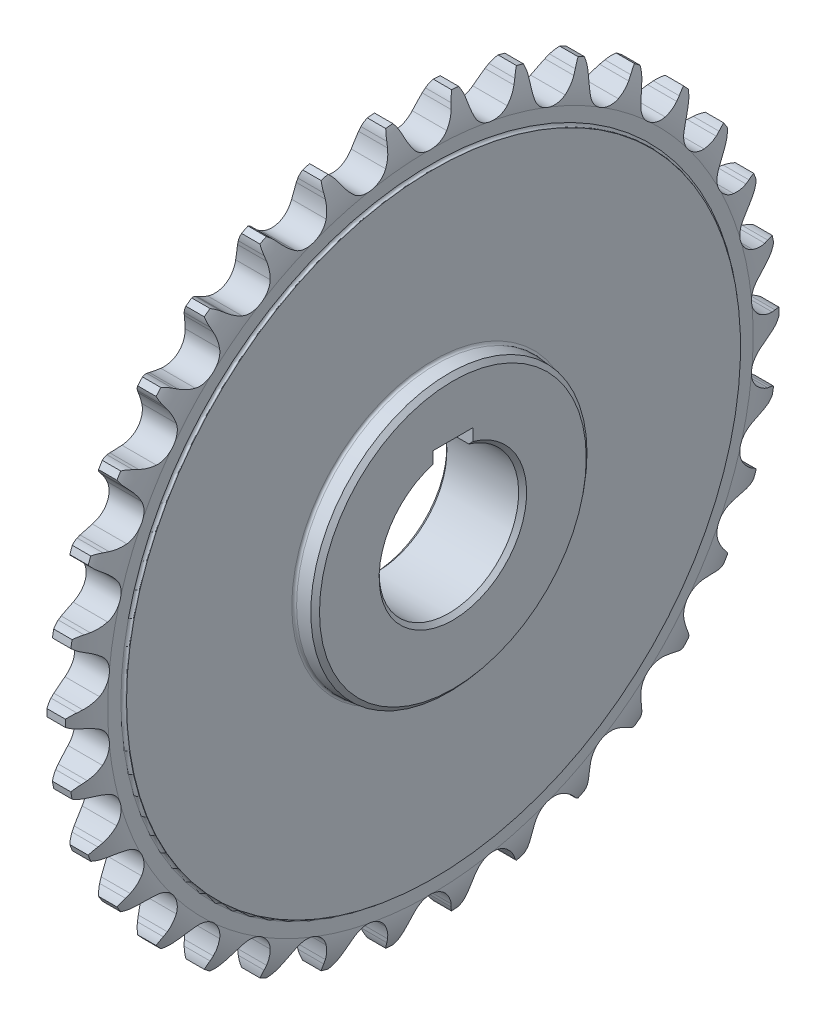
from build123d import *
from OCP.BRepFilletAPI import BRepFilletAPI_MakeChamfer

# Parameters (mm, degrees)
CUT_EXTRUDE_1_DEPTH      = 5.15
PATTERN_CIRCULAR_1_COUNT = 34
SKETCH_4_W               = 10
SKETCH_4_H               = 4.029490121
CUT_EXTRUDE_2_DEPTH      = 128.262907118
FILLET_1_R               = 0.635
CHAMFER_1_SIZE           = 1
CHAMFER_1_SIZE2          = 1.100062868


with BuildPart() as part:
    # 草图1 → 旋转1 (revolve)
    with BuildSketch(Plane.XY, mode=Mode.PRIVATE) as revolve_1_sk:
        with BuildLine():
            Line((-5.15, 17.5), (-5.15, 77))
            Line((-5.15, 77), (-5.006, 77))
            ThreePointArc((-5.006, 77), (-4.556987194, 77.185987194), (-4.371, 77.635))
            Line((-4.371, 77.635), (-4.371, 80.946239614))
            ThreePointArc((-4.371, 80.946239614), (-3.943611485, 85.368963147), (-2.30725, 89.5))
            Line((-2.30725, 89.5), (2.30725, 89.5))
            ThreePointArc((2.30725, 89.5), (3.943611485, 85.368963147), (4.371, 80.946239614))
            Line((4.371, 80.946239614), (4.371, 77.635))
            ThreePointArc((4.371, 77.635), (4.556987194, 77.185987194), (5.006, 77))
            Line((5.006, 77), (5.15, 77))
            Line((5.15, 77), (5.15, 17.5))
            Line((5.15, 17.5), (-5.15, 17.5))
        make_face()
    revolve(revolve_1_sk.sketch.rotate(Axis((-7.9375, 0, 0), (1, 0, 0)), 90), axis=Axis((-7.9375, 0, 0), (1, 0, 0)))

    # 草图2 → 切除-拉伸1 (cut, symmetric)
    with BuildSketch(Plane(origin=(0, 0, 0), x_dir=(0, 0, -1), z_dir=(1, 0, 0))):
        with BuildLine():
            Line((5.937998019, 86.258315079), (6.34124112, 87.341922018))
            ThreePointArc((6.34124112, 87.341922018), (6.78291151, 88.306679102), (7.360367351, 89.196832861))
            ThreePointArc((7.360367351, 89.196832861), (0, 89.5), (-7.360367351, 89.196832861))
            ThreePointArc((-7.360367351, 89.196832861), (-6.78291151, 88.306679102), (-6.34124112, 87.341922018))
            Line((-6.34124112, 87.341922018), (-5.937998019, 86.258315079))
            ThreePointArc((-5.937998019, 86.258315079), (-5.15256189, 84.534832792), (-4.129992057, 82.940576838))
            ThreePointArc((-4.129992057, 82.940576838), (0, 80.870839614), (4.129992057, 82.940576838))
            ThreePointArc((4.129992057, 82.940576838), (5.15256189, 84.534832792), (5.937998019, 86.258315079))
        make_face()
    cut_extrude_1 = extrude(amount=CUT_EXTRUDE_1_DEPTH, both=True, mode=Mode.SUBTRACT)

    # 阵列(圆周)1: 切除-拉伸1 ×34 about axis
    pattern_circular_1_axis = Axis((0, 0, 0), (1, 0, 0))
    for i in range(1, PATTERN_CIRCULAR_1_COUNT):
        add(cut_extrude_1.rotate(pattern_circular_1_axis, i * 360 / PATTERN_CIRCULAR_1_COUNT), mode=Mode.SUBTRACT)

    # 草图5 → 旋转2 (revolve)
    with BuildSketch(Plane.XY, mode=Mode.PRIVATE) as revolve_2_sk:
        Polygon((-10, 17.5), (10, 17.5), (10, 34.553858126), (5.15, 34.978178144), (-5.15, 34.978178144), (-10, 34.553858126), align=None)
    revolve(revolve_2_sk.sketch.rotate(Axis((0, 0, 0), (-1, 0, 0)), 90), axis=Axis((0, 0, 0), (-1, 0, 0)))

    # 草图4 → 切除-拉伸2 (cut, through all)
    with BuildSketch(Plane.ZY.offset(5.15)):
        with Locations((0, 18.785254892)):
            Rectangle(SKETCH_4_W, SKETCH_4_H)
    cut_extrude_2 = extrude(amount=-CUT_EXTRUDE_2_DEPTH, mode=Mode.SUBTRACT)

    # 镜向1: 切除-拉伸2 across plane
    add(cut_extrude_2.mirror(Plane(origin=(0, 0, 0), x_dir=(0, 0, 1), z_dir=(1, 0, 0))), mode=Mode.SUBTRACT)

    # 圆角1
    fillet_1_edges = [part.edges().sort_by_distance(p)[0] for p in [
        (-5.15, 0, 34.978178144),
        (5.15, 0, 34.978178144),
    ]]
    fillet(fillet_1_edges, radius=FILLET_1_R)

    # 倒角1: one chamfer whose edges measure the first distance from different faces: ONE call of the kernel's chamfer builder (chamfer() names one face for all edges)
    chamfer_1_edges_1 = [part.edges().sort_by_distance(p)[0] for p in [
        (-10, 0, 34.553858126),
    ]]
    chamfer_1_side_1 = [part.faces().sort_by_distance(p)[0] for p in [
        (-10, 0, 33.57652743),
    ]]
    chamfer_1_edges_2 = [part.edges().sort_by_distance(p)[0] for p in [
        (10, 0, 34.553858126),
    ]]
    chamfer_1_side_2 = [part.faces().sort_by_distance(p)[0] for p in [
        (7.864828052, 0, 34.740661466),
    ]]
    chamfer_1_edges_3 = [part.edges().sort_by_distance(p)[0] for p in [
        (10, -17.5, 0),
        (-10, -17.5, 0),
    ]]
    chamfer_1 = BRepFilletAPI_MakeChamfer(part.part.solid().wrapped)
    for e in chamfer_1_edges_1:
        chamfer_1.Add(CHAMFER_1_SIZE, CHAMFER_1_SIZE2, e.wrapped, chamfer_1_side_1[0].wrapped)  # the first distance lies on this face
    for e in chamfer_1_edges_2:
        chamfer_1.Add(CHAMFER_1_SIZE, CHAMFER_1_SIZE2, e.wrapped, chamfer_1_side_2[0].wrapped)  # the first distance lies on this face
    for e in chamfer_1_edges_3:
        chamfer_1.Add(CHAMFER_1_SIZE, e.wrapped)
    add(Compound.cast(chamfer_1.Shape()), mode=Mode.REPLACE)


solid = part.part
